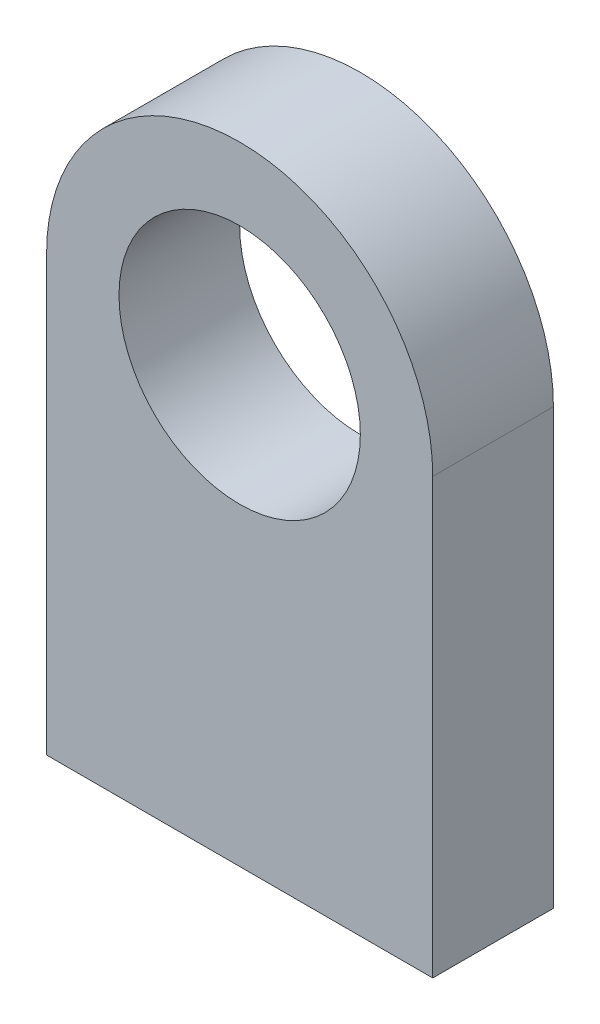
SolidWorks part; units mm, degrees
ref_plane "前视基准面" through (0, 0, 0) normal (0, 0, 1) x (1, 0, 0)
ref_plane "上视基准面" through (0, 0, 0) normal (0, 1, 0) x (1, 0, 0)
ref_plane "右视基准面" through (0, 0, 0) normal (1, 0, 0) x (0, 0, -1)
sketch "草图1" plane through (0, 0, 0) normal (0, 0, 1) x (1, 0, 0)
  line L0 (8, 0) -> (8, 18)
  line L1 (55, 0) -> (-55, 0) construction
  line L3 (-8, 18) -> (-8, 0)
  line L4 (-8, 0) -> (8, 0)
  line L5 (0, 76.7192) -> (0, -59.7374) construction
  line L6 (0, -55) -> (0, 55) construction
  arc A0 (8, 18) -> (-8, 18) centre (0, 18) ccw
  circle A1 centre (0, 18) radius 5
  dimension "D3" = 10
  dimension "D4" = 18
  dimension "D1" = 16
  dimension "D2" = 18
extrude "凸台-拉伸1" add sketch "草图1" along normal mid plane 5
